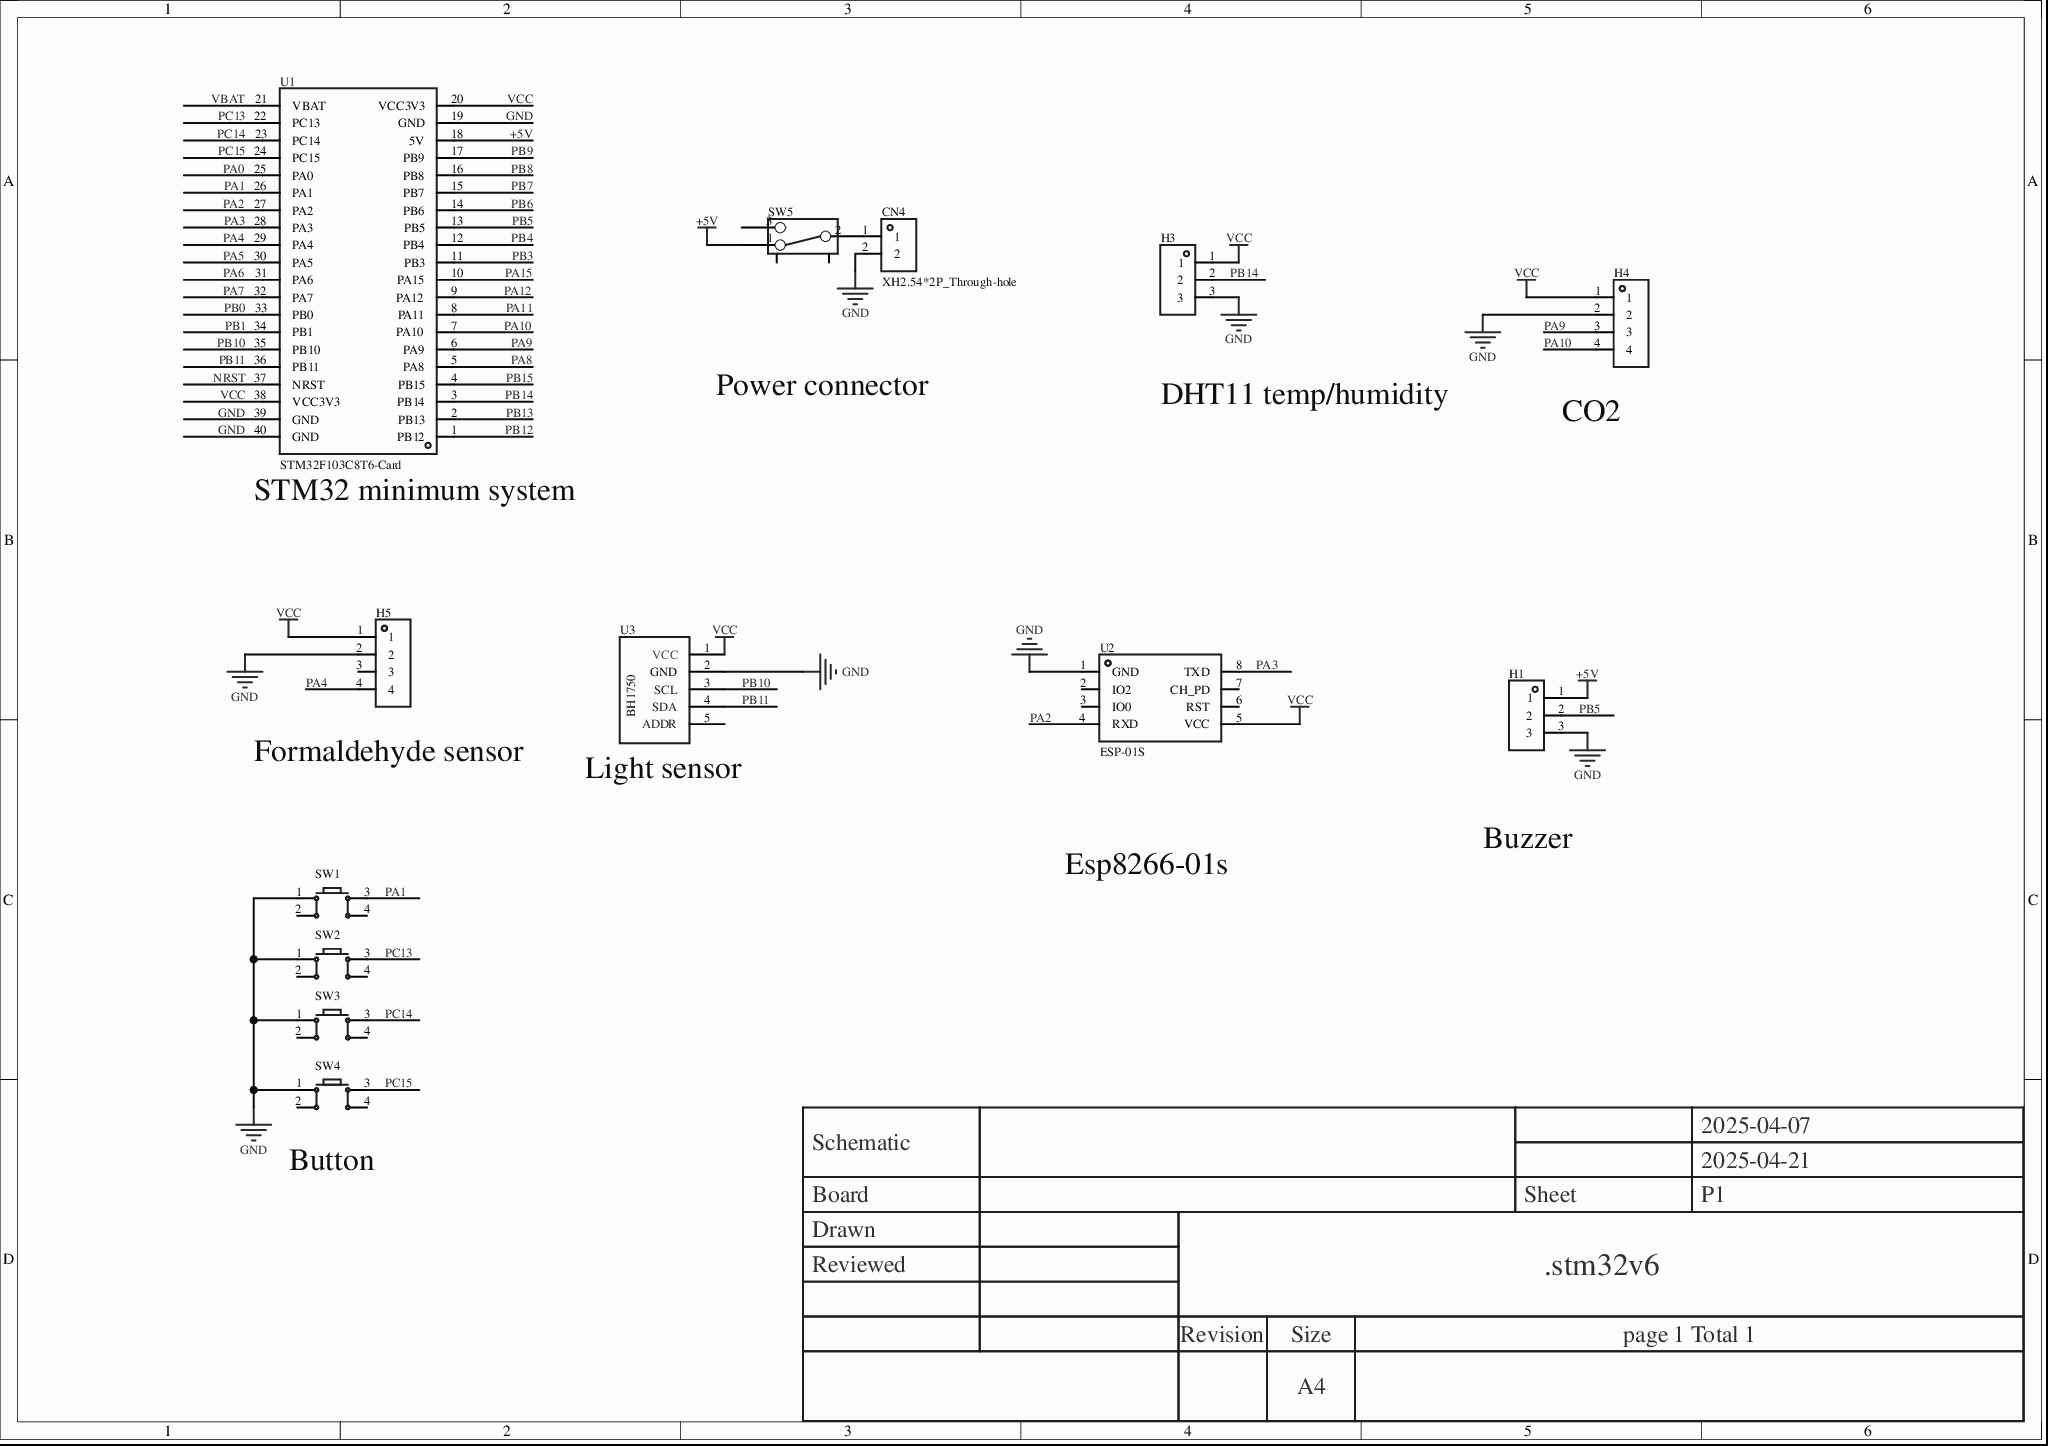
[diagram p0: MISC51847-3.schdoc]
# Altium project MISC51847-2.PrjPcb
1 sheet, 13 parts. Net scope: global (net labels, ports and power ports of the same name join across sheets).
Board file: MISC51847.pcbdoc

## Sheet MISC51847-3.schdoc
size 297 x 209 mm; Version: V1.0; @Project Name: MISC51847; @Page Count: 1; @Update Date: 2026-04-16; @Create Date: 2026-04-16; @Schematic Name: MISC51847; @Page No: 1; @Create Time: 23:22:16; @Update Time: 17:32:40; @Board Name: MISC51847

### Parts
CN4  XH2.54*2P_Through-hole  [CONN-TH_2P-P2.50-XH2.54-2P]
H1  (no value)  [HDR-TH_3P-P2.54-V-F]
H3  (no value)  [HDR-TH_3P-P2.54-V-F]
H4  (no value)  [HDR-TH_4P-P2.54-V-F]
H5  (no value)  [HDR-TH_4P-P2.54-V-F]
SW1  (no value)  [SW-TH_4P-L6.0-W6.0-P4.50-LS6.5]
SW2  (no value)  [SW-TH_4P-L6.0-W6.0-P4.50-LS6.5]
SW3  (no value)  [SW-TH_4P-L6.0-W6.0-P4.50-LS6.5]
SW4  (no value)  [SW-TH_4P-L6.0-W6.0-P4.50-LS6.5]
SW5  (no value)  [拨动开关]
U1  STM32F103C8T6-Card  [CONN-TH_L53.3-W22.9_STM32F103C8T6-CARD]
U2  ESP-01S  [WIFIM-TH_ESP-01S]
U3  (no value)  [BH1750光照传感器]

### Nets
+5V: H1.1 SW5.1 U1.18(5V)
GND: CN4.2 H1.3 H3.3 H4.2 H5.2 SW1.1 SW2.1 SW3.1 SW4.1 U1.19(GND) U1.39(GND) U1.40(GND) U2.1(GND) U3.2(GND)
VCC: H3.1 H4.1 H5.1 U1.20(VCC3V3) U1.38(VCC3V3) U2.5(VCC) U3.1(VCC)
NRST: U1.37(NRST)
PA0: U1.25(PA0)
PA1: SW1.3 U1.26(PA1)
PA2: U1.27(PA2) U2.4(RXD)
PA3: U1.28(PA3) U2.8(TXD)
PA4: H5.4 U1.29(PA4)
PA5: U1.30(PA5)
PA6: U1.31(PA6)
PA7: U1.32(PA7)
PA8: U1.5(PA8)
PA9: H4.3 U1.6(PA9)
PA10: H4.4 U1.7(PA10)
PA11: U1.8(PA11)
PA12: U1.9(PA12)
PA15: U1.10(PA15)
PB0: U1.33(PB0)
PB1: U1.34(PB1)
PB3: U1.11(PB3)
PB4: U1.12(PB4)
PB5: H1.2 U1.13(PB5)
PB6: U1.14(PB6)
PB7: U1.15(PB7)
PB8: U1.16(PB8)
PB9: U1.17(PB9)
PB10: U1.35(PB10) U3.3(SCL)
PB11: U1.36(PB11) U3.4(SDA)
PB12: U1.1(PB12)
PB13: U1.2(PB13)
PB14: H3.2 U1.3(PB14)
PB15: U1.4(PB15)
PC13: SW2.3 U1.22(PC13)
PC14: SW3.3 U1.23(PC14)
PC15: SW4.3 U1.24(PC15)
VBAT: U1.21(VBAT)
NetCN4_1: CN4.1 SW5.2

Not connected (* = marked no-connect by the designer): H5 3; SW1 2 4; SW2 2 4; SW3 2 4; SW4 2 4; SW5 3 4 5; U2 2(IO2)* 3(IO0)* 6(RST)* 7(CH_PD)*; U3 5(ADDR)

### Notes on the sheet
- Power connector
- DHT11 temp/humidity
- (near H4) CO2
- (near U1) STM32 minimum system
- (near H5) Formaldehyde sensor
- (near U3) Light sensor
- Buzzer
- Esp8266-01s
- (near SW4) Button
- 2025-04-07
- Schematic
- Board
- Sheet
- 2025-04-21
- P1
- Drawn
- Reviewed
- .stm32v6
- Revision
- Size
- A4
- page 1 Total 1

### Library data of the parts
CN4 = XH2.54*2P_直插: 3D Model: 325c595e30db4df8abe76612dd40b0fa0819f05c4eef4c71ace90d822a990e87; 3D Model Transform: 295.275,228.346,0,180,0,0,-0.002,-20.079,-137.795; AddInBom: yes; Device: XH2.54*2P_Through-hole; Symbol: XH2.54*2P_Through-hole; LCSC Part Name: XH2.54*2P_直插; Supplier Part: C9900008615; Manufacturer Part: XH2.54*2P_直插; Supplier Footprint: XH2.54_2P; JLCPCB Part Class: Extended Part; Supplier: LCSC; FootprintName: CONN-TH_2P-P2.50-XH2.54-2P; ConvertToPcb: yes; ModelName: CONN-TH_2P-P2.50-XH2.54-2P
H1 H3 = HDR-F_2.54_1x3P: Symbol: PM254V-11-03-H85; 3D Model: f3b3cc5aae9641bf9e56fc160cef875b; 3D Model Transform: 299.9994,100,0,0,0,0,0,0,-118.11; ConvertToPcb: yes; ModelName: HDR2.54-F-LI-1X3P; Device: HDR-F_2.54_1x3P; Supplier Part: C541850; Supplier Footprint: 插件; FootprintName: HDR-TH_3P-P2.54-V-F; AddInBom: yes
H4 = HDR-F_2.54_1x4P: Symbol: 2.54-1*4P female; ConvertToPcb: yes; ModelId: d187812051054f85879fcaa51a310d8e0819f05c4eef4c71ace90d822a990e87; ModelTransform: 419.6842,98.464,0,0,0,0,0,0,-118.11; Device: HDR-F_2.54_1x4P; FootprintName: HDR-TH_4P-P2.54-V-F; AddInBom: yes; SupplierPart: C2718488; Supplier Footprint: 插件; ModelName: HDR-TH_4P-P2.54-V-F
H5 = HDR-F_2.54_1x4P: Symbol: 2.54-1*4P female; 3D Model: d187812051054f85879fcaa51a310d8e0819f05c4eef4c71ace90d822a990e87; 3D Model Transform: 419.6842,98.464,0,0,0,0,0,0,-118.11; ConvertToPcb: yes; Device: HDR-F_2.54_1x4P; Supplier Part: C2718488; Supplier Footprint: 插件; FootprintName: HDR-TH_4P-P2.54-V-F; AddInBom: yes; ModelName: HDR-TH_4P-P2.54-V-F
SW1-SW4 = Key_TH_6x6x6: 触点电流:50mA;额定电压(DC):12V;绝缘电阻:100MΩ;电路结构:单刀单掷;安装方式:直插;按钮形状:圆形按钮;按钮/盖帽颜色:黑色;作用力:260gf@±30gf;工作温度:-25℃~+70℃;引脚样式:PC引脚;开关长度:6mm;开关宽度:6mm;开关高度:6mm;带支架:否;; Symbol: Tactile switch; AddInBom: yes; ModelId: 20eee248bc684ccd8cbdbb1d0d91ec6f0819f05c4eef4c71ace90d822a990e87; ModelName: SW-TH_4P-L6.0-W6.0-H5.0-LS6.5-P4.50; ModelTransform: 236.22,323.03,0,90,0,0,0,0,-137.795; Device: Key_TH_6x6x6; FootprintName: SW-TH_4P-L6.0-W6.0-P4.50-LS6.5; ConvertToPcb: yes; Supplier Footprint: 插件
SW5 = 拨动开关_正: Device: Toggle switch_pos; Symbol: Toggle switch; ConvertToPcb: yes; ModelId: 4321fe59a4074cbfb4989553f297c68f0819f05c4eef4c71ace90d822a990e87; ModelName: SW-TH_SS-12D02-VG4; ModelTransform: 370.09,208.7,472.35,0,0,0,0,0,-110; FootprintName: Toggle switch; AddInBom: yes; Supplier Footprint: 插件
U1 = STM32F103C8T6-Card: AddInBom: yes; Device: STM32F103C8T6-Card; Symbol: STM32F103C8T6-CARD; FootprintName: CONN-TH_L53.3-W22.9_STM32F103C8T6-CARD; LCSC Part Name: STM32F103C8T6-Card; SupplierPart: C9900077949; ManufacturerPart: STM32F103C8T6-Card; Supplier Footprint: 插件; Supplier: LCSC; ConvertToPcb: yes
U2 = ESP-01S_C111009: 3D Model: eb7175da78ae48b3b1568cfe3027405f0819f05c4eef4c71ace90d822a990e87; 3D Model Transform: 582.676,976.37608,0,0,0,0,0,388.346,-118.11; AddInBom: yes; Symbol: ESP-01S; Device: ESP-01S_C111009; LCSC Part Name: ESP-01S; Supplier Part: C111009; Manufacturer Part: ESP-01S; Supplier Footprint: -; JLCPCB Part Class: Extended Part; Supplier: LCSC; ConvertToPcb: yes; FootprintName: WIFIM-TH_ESP-01S; ModelName: WIFIM-TH_ESP-01S
U3 = BH1750光照传感器: Symbol: BH1750 light sensor; AddInBom: yes; Device: BH1750 light sensor; ConvertToPcb: yes; FootprintName: BH1750 light sensor